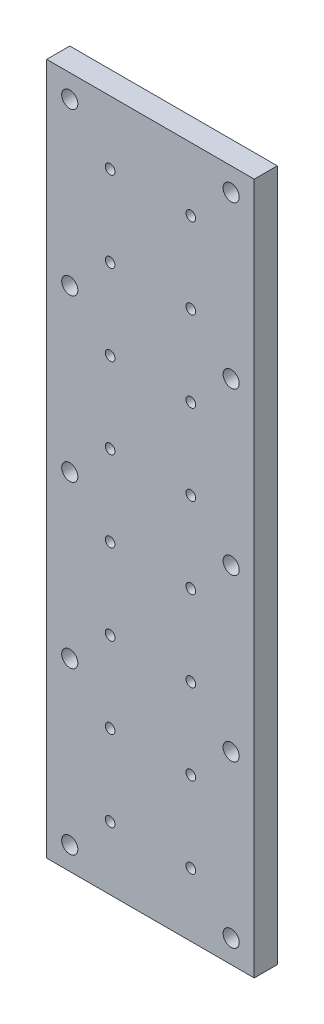
from build123d import *

# Parameters (mm, degrees)
SKETCH1_W                = 90
SKETCH1_H                = 300
BOSS_EXTRUDE1_DEPTH      = 10
F_7_0_7_DIAMETER_HOLE1_D = 7
LPATTERN1_COUNT          = 3
LPATTERN1_PITCH          = 70
LPATTERN1_COUNT_DIR2     = 2
LPATTERN1_PITCH_DIR2     = 70
LPATTERN2_COUNT          = 3
LPATTERN2_PITCH          = 70
LPATTERN2_COPY_1_D       = 7
LPATTERN2_COPY_2_D       = 7
LPATTERN2_COPY_3_D       = 7
LPATTERN2_COPY_4_D       = 7
LPATTERN2_COPY_5_D       = 7
LPATTERN2_COPY_6_D       = 7
LPATTERN2_COPY_7_D       = 7
LPATTERN2_COPY_8_D       = 7
LPATTERN2_COPY_9_D       = 7
LPATTERN2_COPY_10_D      = 7
M5_TAPPED_HOLE1_D        = 4.2
LPATTERN3_COUNT          = 4
LPATTERN3_PITCH          = 35
LPATTERN3_COL_COUNT      = 4
LPATTERN3_COL_PITCH      = 35


with BuildPart() as part:
    # Sketch1 → Boss-Extrude1 (new body)
    with BuildSketch(Plane.XY):
        Rectangle(SKETCH1_W, SKETCH1_H)
    extrude(amount=BOSS_EXTRUDE1_DEPTH)

    # Ø7.0 (7) Diameter Hole1 (through all)
    with Locations(Plane.XY.offset(10)):
        with Locations((-35, 0)):
            f_7_0_7_diameter_hole1 = Hole(F_7_0_7_DIAMETER_HOLE1_D / 2)

    # LPattern1: 7.0 _7_ Diameter Hole1 3 × 2
    with Locations(*[(j * LPATTERN1_PITCH_DIR2, -i * LPATTERN1_PITCH, 0) for i in range(LPATTERN1_COUNT) for j in range(LPATTERN1_COUNT_DIR2) if (i, j) != (0, 0)]):
        add(f_7_0_7_diameter_hole1, mode=Mode.SUBTRACT)

    # LPattern2: Ø7.0 (7) Diameter Hole1 ×3
    with Locations(*[(0, i * LPATTERN2_PITCH, 0) for i in range(1, LPATTERN2_COUNT)]):
        add(f_7_0_7_diameter_hole1, mode=Mode.SUBTRACT)

    # LPattern2 copy 1 (through all)
    with Locations(Plane(origin=(70, 70, 10), x_dir=(1, 0, 0), z_dir=(0, 0, 1))):
        with Locations((-35, 0)):
            Hole(LPATTERN2_COPY_1_D / 2)

    # LPattern2 copy 2 (through all)
    with Locations(Plane(origin=(70, 140, 10), x_dir=(1, 0, 0), z_dir=(0, 0, 1))):
        with Locations((-35, 0)):
            Hole(LPATTERN2_COPY_2_D / 2)

    # LPattern2 copy 3 (through all)
    with Locations(Plane.XY.offset(10)):
        with Locations((-35, 0)):
            Hole(LPATTERN2_COPY_3_D / 2)

    # LPattern2 copy 4 (through all)
    with Locations(Plane(origin=(0, 70, 10), x_dir=(1, 0, 0), z_dir=(0, 0, 1))):
        with Locations((-35, 0)):
            Hole(LPATTERN2_COPY_4_D / 2)

    # LPattern2 copy 5 (through all)
    with Locations(Plane(origin=(70, 0, 10), x_dir=(1, 0, 0), z_dir=(0, 0, 1))):
        with Locations((-35, 0)):
            Hole(LPATTERN2_COPY_5_D / 2)

    # LPattern2 copy 6 (through all)
    with Locations(Plane(origin=(70, 70, 10), x_dir=(1, 0, 0), z_dir=(0, 0, 1))):
        with Locations((-35, 0)):
            Hole(LPATTERN2_COPY_6_D / 2)

    # LPattern2 copy 7 (through all)
    with Locations(Plane(origin=(0, -70, 10), x_dir=(1, 0, 0), z_dir=(0, 0, 1))):
        with Locations((-35, 0)):
            Hole(LPATTERN2_COPY_7_D / 2)

    # LPattern2 copy 8 (through all)
    with Locations(Plane.XY.offset(10)):
        with Locations((-35, 0)):
            Hole(LPATTERN2_COPY_8_D / 2)

    # LPattern2 copy 9 (through all)
    with Locations(Plane(origin=(70, -70, 10), x_dir=(1, 0, 0), z_dir=(0, 0, 1))):
        with Locations((-35, 0)):
            Hole(LPATTERN2_COPY_9_D / 2)

    # LPattern2 copy 10 (through all)
    with Locations(Plane(origin=(70, 0, 10), x_dir=(1, 0, 0), z_dir=(0, 0, 1))):
        with Locations((-35, 0)):
            Hole(LPATTERN2_COPY_10_D / 2)

    # M5 Tapped Hole1 (through all)
    with Locations(Plane(origin=(0, 0, 0), x_dir=(-1, 0, 0), z_dir=(0, 0, -1))):
        with Locations((17.5, 17.5), (17.5, -17.5), (-17.5, -17.5), (-17.5, 17.5)):
            m5_tapped_hole1 = Hole(M5_TAPPED_HOLE1_D / 2)

    # LPattern3: M5 Tapped Hole1 ×4
    with Locations(*[(0, -i * LPATTERN3_PITCH, 0) for i in range(1, LPATTERN3_COUNT)]):
        add(m5_tapped_hole1, mode=Mode.SUBTRACT)

    # LPattern3 col: M5 Tapped Hole1 ×4
    with Locations(*[(0, i * LPATTERN3_COL_PITCH, 0) for i in range(1, LPATTERN3_COL_COUNT)]):
        add(m5_tapped_hole1, mode=Mode.SUBTRACT)


solid = part.part
